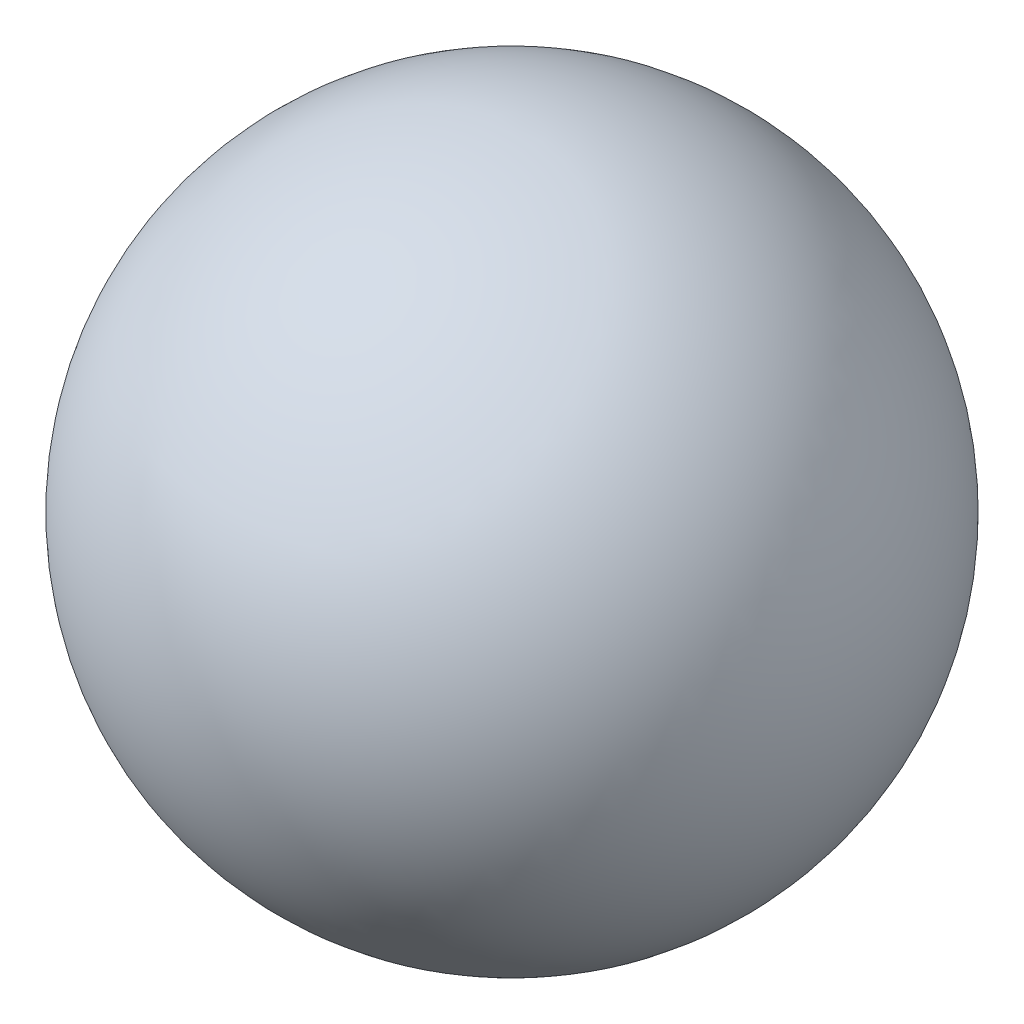
SolidWorks part; units mm, degrees
ref_plane "Front Plane" through (0, 0, 0) normal (0, 0, 1) x (1, 0, 0)
ref_plane "Top Plane" through (0, 0, 0) normal (0, 1, 0) x (1, 0, 0)
ref_plane "Right Plane" through (0, 0, 0) normal (1, 0, 0) x (0, 0, -1)
other "Configuration Table"
sketch "Sketch1" plane through (0, 0, 0) normal (0, 0, 1) x (1, 0, 0)
  line L0 (0, 0) -> (0, 5.5) construction
  line L1 (0, 0) -> (0, 5.5)
  arc A0 (0, 5.5) -> (0, 0) centre (0, 2.75) ccw
  dimension "D1" = 2.75
revolve "Revolve1" add sketch "Sketch1" angle 360 about L0
